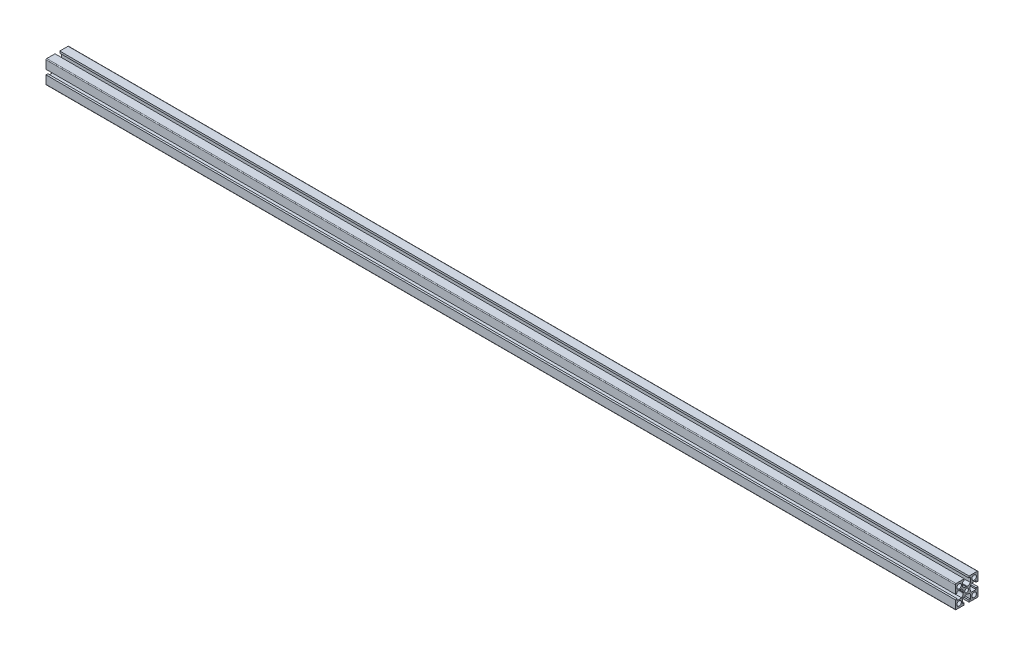
from build123d import *

# Parameters (mm, degrees)
SKETCH_11_R         = 3
SKETCH_11_R_2       = 2.5
F_0_GY_3030_1_DEPTH = 1200


with BuildPart() as part:
    # 草图11 → 0国耀铝型材 GY-3030国标铝型材(1) (new body)
    with BuildSketch(Plane.YZ):
        with BuildLine():
            Line((-14, -15), (-3.15, -15))
            Line((-3.15, -15), (-3.15, -12.5))
            Line((-3.15, -12.5), (-5.15, -12.5))
            Line((-5.15, -12.5), (-5.15, -6.5))
            ThreePointArc((-5.15, -6.5), (-3.019390742, -5.122695475), (-0.555, -4.52))
            Line((-0.555, -4.52), (0, -4.2))
            Line((0, -4.2), (0.555, -4.52))
            ThreePointArc((0.555, -4.52), (3.019390742, -5.122695475), (5.15, -6.5))
            Line((5.15, -6.5), (5.15, -12.5))
            Line((5.15, -12.5), (3.15, -12.5))
            Line((3.15, -12.5), (3.15, -15))
            Line((3.15, -15), (14, -15))
            ThreePointArc((14, -15), (14.707106781, -14.707106781), (15, -14))
            Line((15, -14), (15, -3.15))
            Line((15, -3.15), (12.5, -3.15))
            Line((12.5, -3.15), (12.5, -5.15))
            Line((12.5, -5.15), (6.5, -5.15))
            ThreePointArc((6.5, -5.15), (5.12253592, -3.018923167), (4.52, -0.554))
            Line((4.52, -0.554), (4.2, 0))
            Line((4.2, 0), (4.52, 0.555))
            ThreePointArc((4.52, 0.555), (5.122695475, 3.019390742), (6.5, 5.15))
            Line((6.5, 5.15), (12.5, 5.15))
            Line((12.5, 5.15), (12.5, 3.15))
            Line((12.5, 3.15), (15, 3.15))
            Line((15, 3.15), (15, 14))
            ThreePointArc((15, 14), (14.707106781, 14.707106781), (14, 15))
            Line((14, 15), (3.15, 15))
            Line((3.15, 15), (3.15, 12.5))
            Line((3.15, 12.5), (5.15, 12.5))
            Line((5.15, 12.5), (5.15, 6.5))
            ThreePointArc((5.15, 6.5), (3.019292492, 5.123227892), (0.555, 4.521))
            Line((0.555, 4.521), (0, 4.2))
            Line((0, 4.2), (-0.555, 4.521))
            ThreePointArc((-0.555, 4.521), (-3.019292492, 5.123227892), (-5.15, 6.5))
            Line((-5.15, 6.5), (-5.15, 12.5))
            Line((-5.15, 12.5), (-3.15, 12.5))
            Line((-3.15, 12.5), (-3.15, 15))
            Line((-3.15, 15), (-14, 15))
            ThreePointArc((-14, 15), (-14.707106781, 14.707106781), (-15, 14))
            Line((-15, 14), (-15, 3.15))
            Line((-15, 3.15), (-12.5, 3.15))
            Line((-12.5, 3.15), (-12.5, 5.15))
            Line((-12.5, 5.15), (-6.5, 5.15))
            ThreePointArc((-6.5, 5.15), (-5.122695475, 3.019390742), (-4.52, 0.555))
            Line((-4.52, 0.555), (-4.2, 0))
            Line((-4.2, 0), (-4.52, -0.554))
            ThreePointArc((-4.52, -0.554), (-5.12253592, -3.018923167), (-6.5, -5.15))
            Line((-6.5, -5.15), (-12.5, -5.15))
            Line((-12.5, -5.15), (-12.5, -3.15))
            Line((-12.5, -3.15), (-15, -3.15))
            Line((-15, -3.15), (-15, -14))
            ThreePointArc((-15, -14), (-14.707106781, -14.707106781), (-14, -15))
        make_face()
        with Locations((9.8, 9.9)):
            Circle(SKETCH_11_R, mode=Mode.SUBTRACT)
        with Locations((9.8, -9.9)):
            Circle(SKETCH_11_R, mode=Mode.SUBTRACT)
        Circle(SKETCH_11_R_2, mode=Mode.SUBTRACT)
        with Locations((-9.8, 9.9)):
            Circle(SKETCH_11_R, mode=Mode.SUBTRACT)
        with Locations((-10, -9.9)):
            Circle(SKETCH_11_R, mode=Mode.SUBTRACT)
    extrude(amount=F_0_GY_3030_1_DEPTH)


solid = part.part
